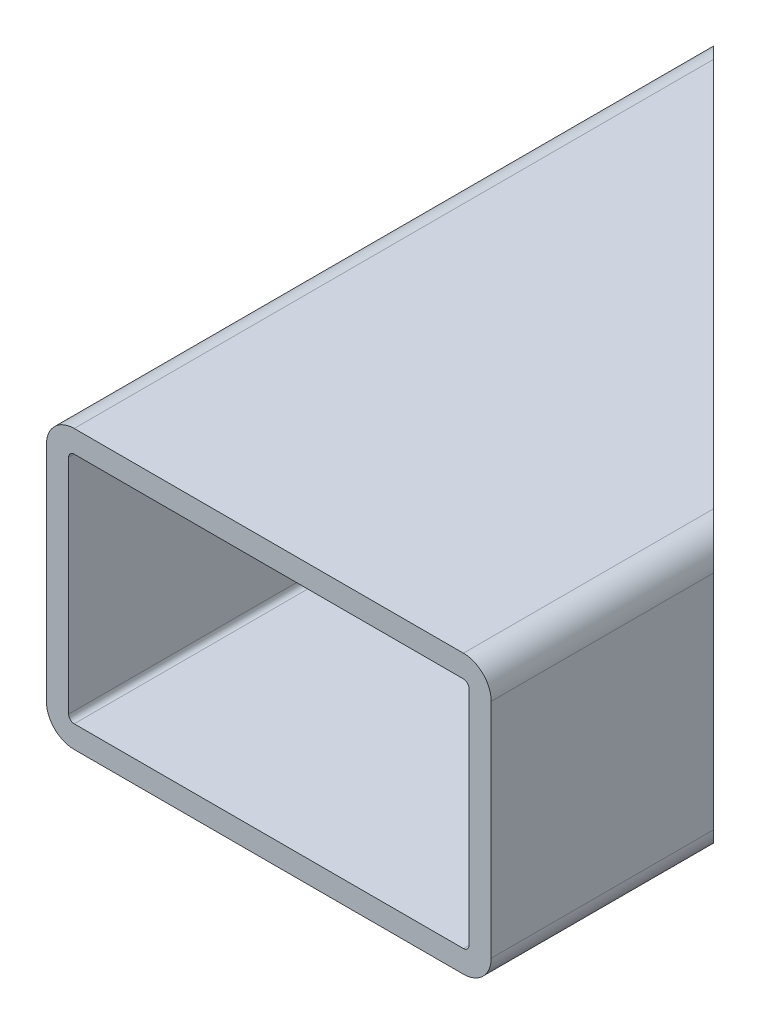
from build123d import *

# Parameters (mm, degrees)
BOSS_EXTRUDE1_DEPTH = 2200
SHELL1_T            = -4
SKETCH2_R           = 3.25
CUT_EXTRUDE1_DEPTH  = 10
CUT_EXTRUDE2_DEPTH  = 2000
SKETCH4_W           = 2035.40419349
SKETCH4_H           = 2143.359963821
CUT_EXTRUDE3_DEPTH  = 2000


with BuildPart() as part:
    # Sketch1 → Boss-Extrude1 (new body)
    with BuildSketch(Plane.XY):
        with BuildLine():
            Line((35, 25), (-35, 25))
            ThreePointArc((-35, 25), (-38.535533906, 23.535533906), (-40, 20))
            Line((-40, 20), (-40, -20))
            ThreePointArc((-40, -20), (-38.535533906, -23.535533906), (-35, -25))
            Line((-35, -25), (35, -25))
            ThreePointArc((35, -25), (38.535533906, -23.535533906), (40, -20))
            Line((40, -20), (40, 20))
            ThreePointArc((40, 20), (38.535533906, 23.535533906), (35, 25))
        make_face()
    extrude(amount=BOSS_EXTRUDE1_DEPTH)

    # Shell1
    shell1_openings = [part.faces().sort_by_distance(p)[0] for p in [
        (0, 0, 2200),
        (0, 0, 0),
    ]]
    offset(amount=SHELL1_T, openings=shell1_openings, kind=Kind.INTERSECTION)

    # Sketch2 → Cut-Extrude1 (cut)
    with BuildSketch(Plane(origin=(0, 25, 0), x_dir=(1, 0, 0), z_dir=(0, 1, 0))):
        with Locations(Location((-25, -919, 0), (0, 0, 180))):
            Circle(SKETCH2_R)
        with Locations(Location((25, -919, 0), (0, 0, 180))):
            Circle(SKETCH2_R)
        with Locations(Location((-25, -849, 0), (0, 0, 180))):
            Circle(SKETCH2_R)
        with Locations(Location((25, -849, 0), (0, 0, 180))):
            Circle(SKETCH2_R)
        with Locations(Location((-25, -1281, 0), (0, 0, 180))):
            Circle(SKETCH2_R)
        with Locations(Location((25, -1281, 0), (0, 0, 180))):
            Circle(SKETCH2_R)
        with Locations(Location((-25, -1351, 0), (0, 0, 180))):
            Circle(SKETCH2_R)
        with Locations(Location((25, -1351, 0), (0, 0, 180))):
            Circle(SKETCH2_R)
    extrude(amount=-CUT_EXTRUDE1_DEPTH, mode=Mode.SUBTRACT)

    # Sketch3 → Cut-Extrude2 (cut)
    with BuildSketch(Plane.XZ.offset(25)):
        Polygon((-40, 2200), (40, 2120), (40, 2200), align=None)
        Polygon((40, 80), (40, 0), (-40, 0), align=None)
    extrude(amount=-CUT_EXTRUDE2_DEPTH, mode=Mode.SUBTRACT)

    # Sketch4 → Cut-Extrude3 (cut)
    with BuildSketch(Plane.XZ.offset(25)):
        with Locations((0, 1191.679981911)):
            Rectangle(SKETCH4_W, SKETCH4_H)
    extrude(amount=-CUT_EXTRUDE3_DEPTH, mode=Mode.SUBTRACT)


solid = part.part
